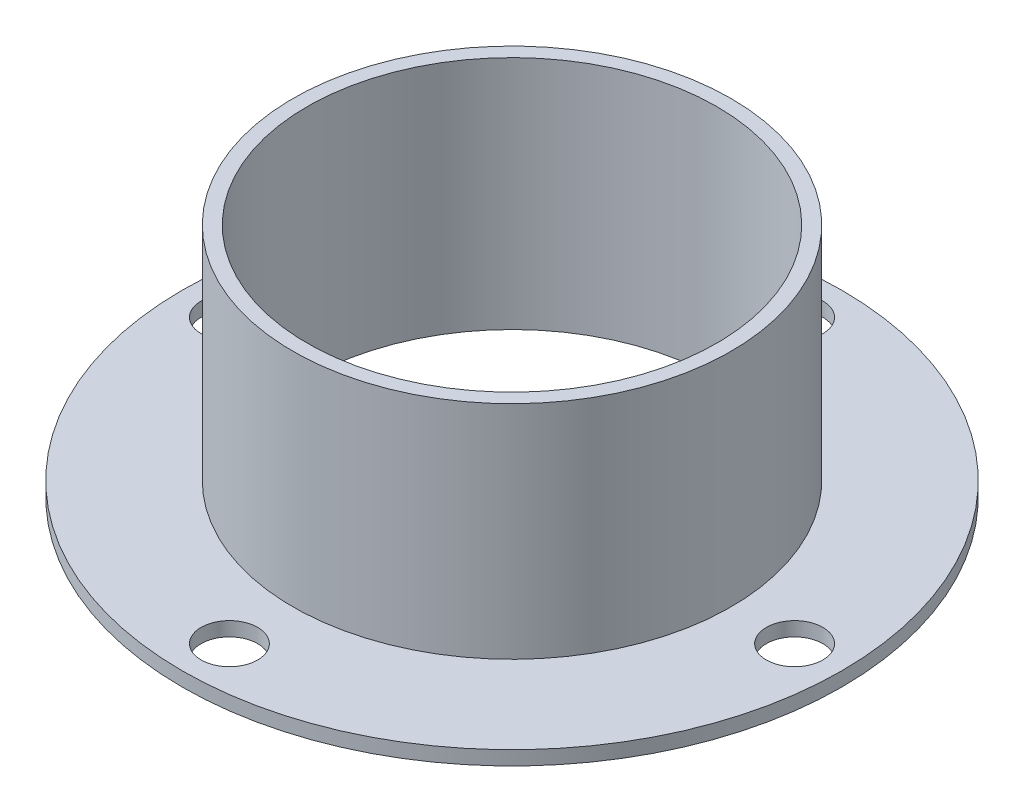
SolidWorks part; units mm, degrees
material "A3"
ref_plane "前视基准面" through (0, 0, 0) normal (0, 0, 1) x (1, 0, 0)
ref_plane "上视基准面" through (0, 0, 0) normal (0, 1, 0) x (1, 0, 0)
ref_plane "右视基准面" through (0, 0, 0) normal (1, 0, 0) x (0, 0, -1)
sketch "草图1" plane through (0, 0, 0) normal (0, 0, 1) x (1, 0, 0)
  line L0 (0, 0) -> (0, 66.5668) construction
  line L1 (43.5, 50) -> (43.5, 0)
  line L2 (43.5, 0) -> (70, 0)
  line L3 (46.5, 50) -> (46.5, 3)
  line L4 (46.5, 3) -> (70, 3)
  line L5 (43.5, 50) -> (46.5, 50)
  line L6 (70, 3) -> (70, 0)
  dimension "D1" = 140
  dimension "D2" = 50
  dimension "D3" = 87
  dimension "D4" = 3
revolve "旋转1" add sketch "草图1" angle 360 about L0
sketch "草图2" plane through (0, 3, 0) normal (0, 1, 0) x (1, 0, 0)
  circle A0 centre (0, 0) radius 60 construction
  circle A1 centre (0, 60) radius 6
  circle A2 centre (60, 0) radius 6
  circle A3 centre (0, -60) radius 6
  circle A4 centre (-60, 0) radius 6
  point P14 (0, 0)
  dimension "D1" = 120
  dimension "D2" = 12
  dimension "D3" = 4
extrude "切除-拉伸1" cut sketch "草图2" against normal through all
